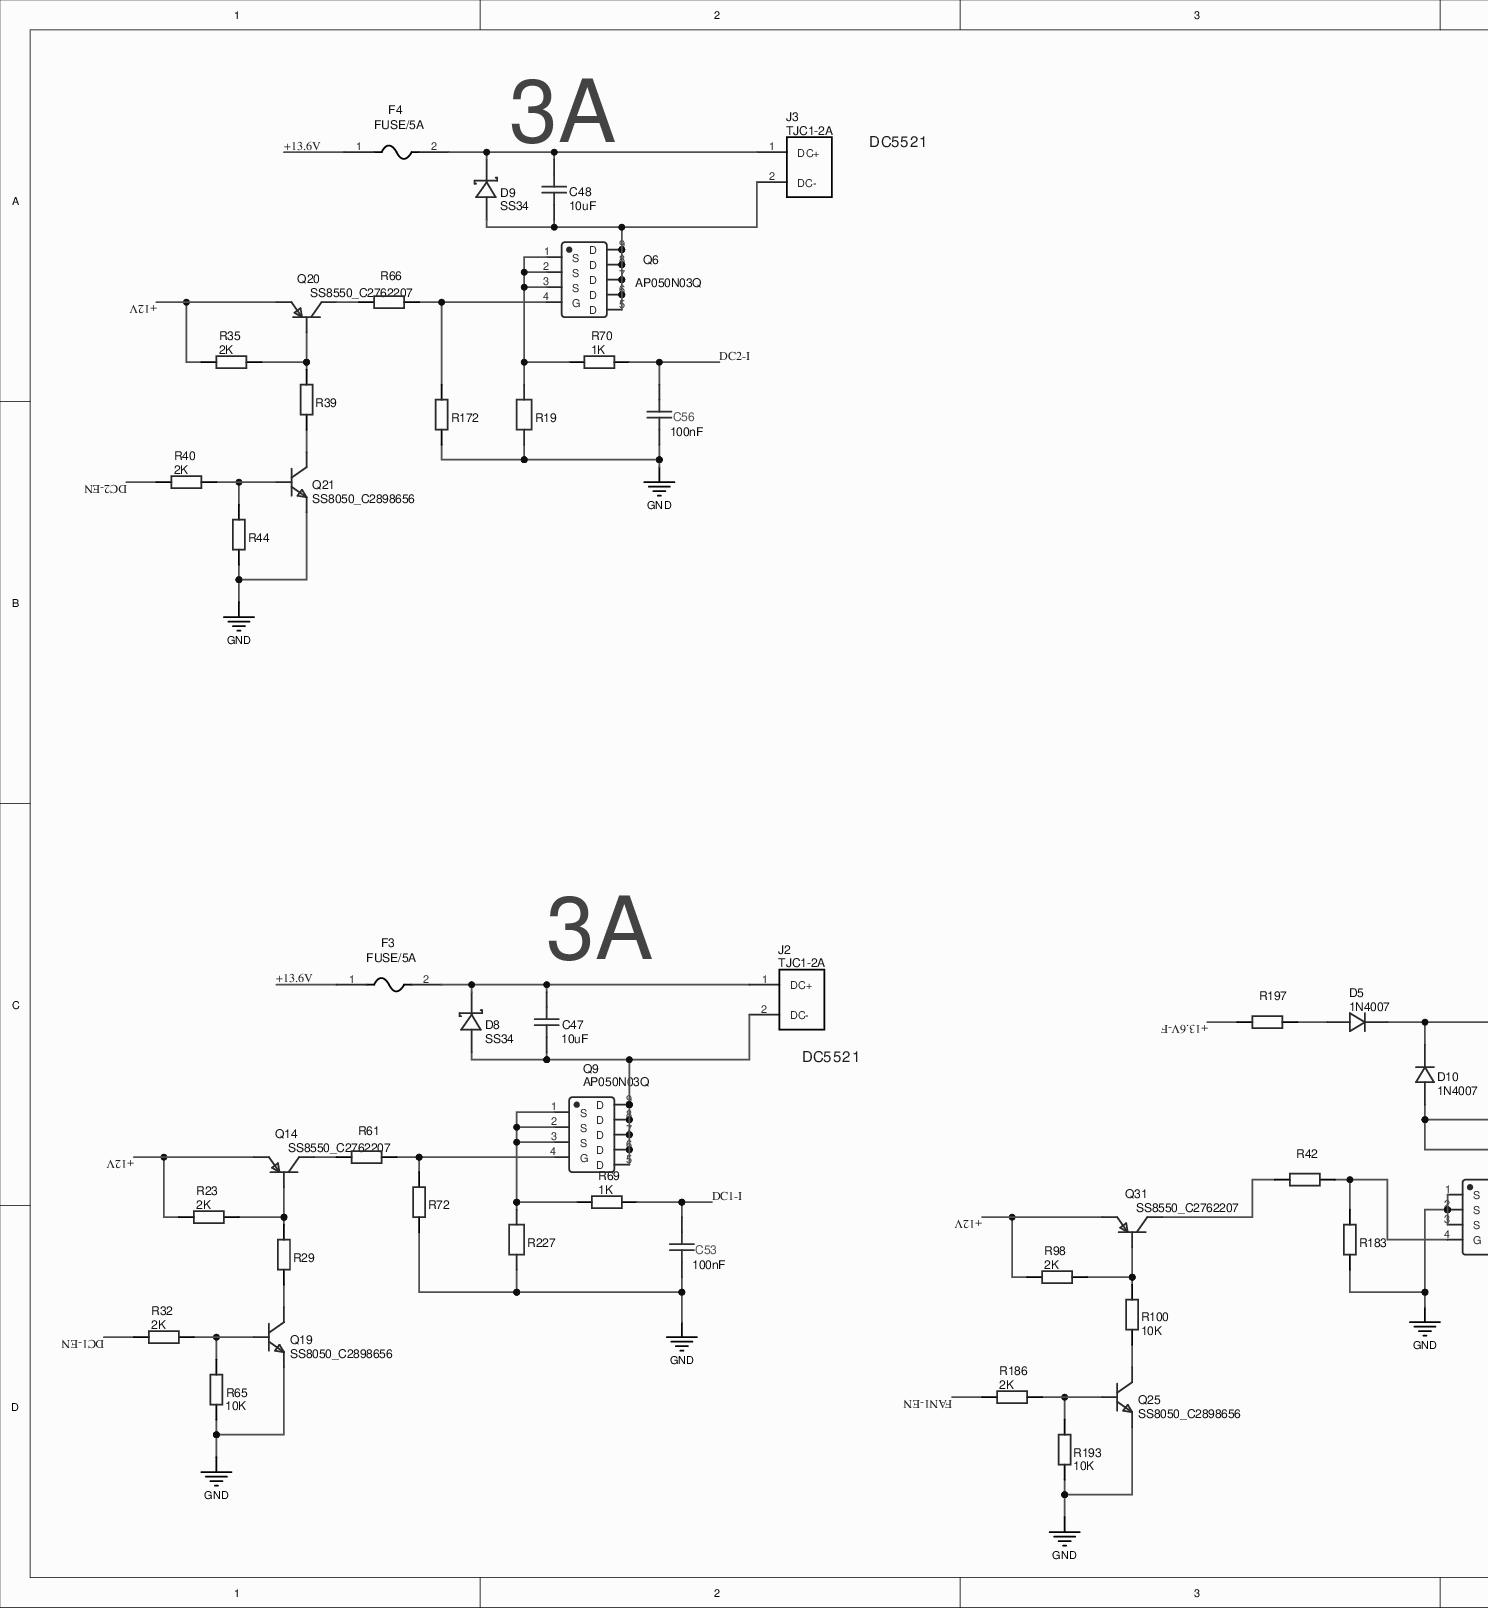
[diagram p0: MISC84402-8.SchDoc, left]
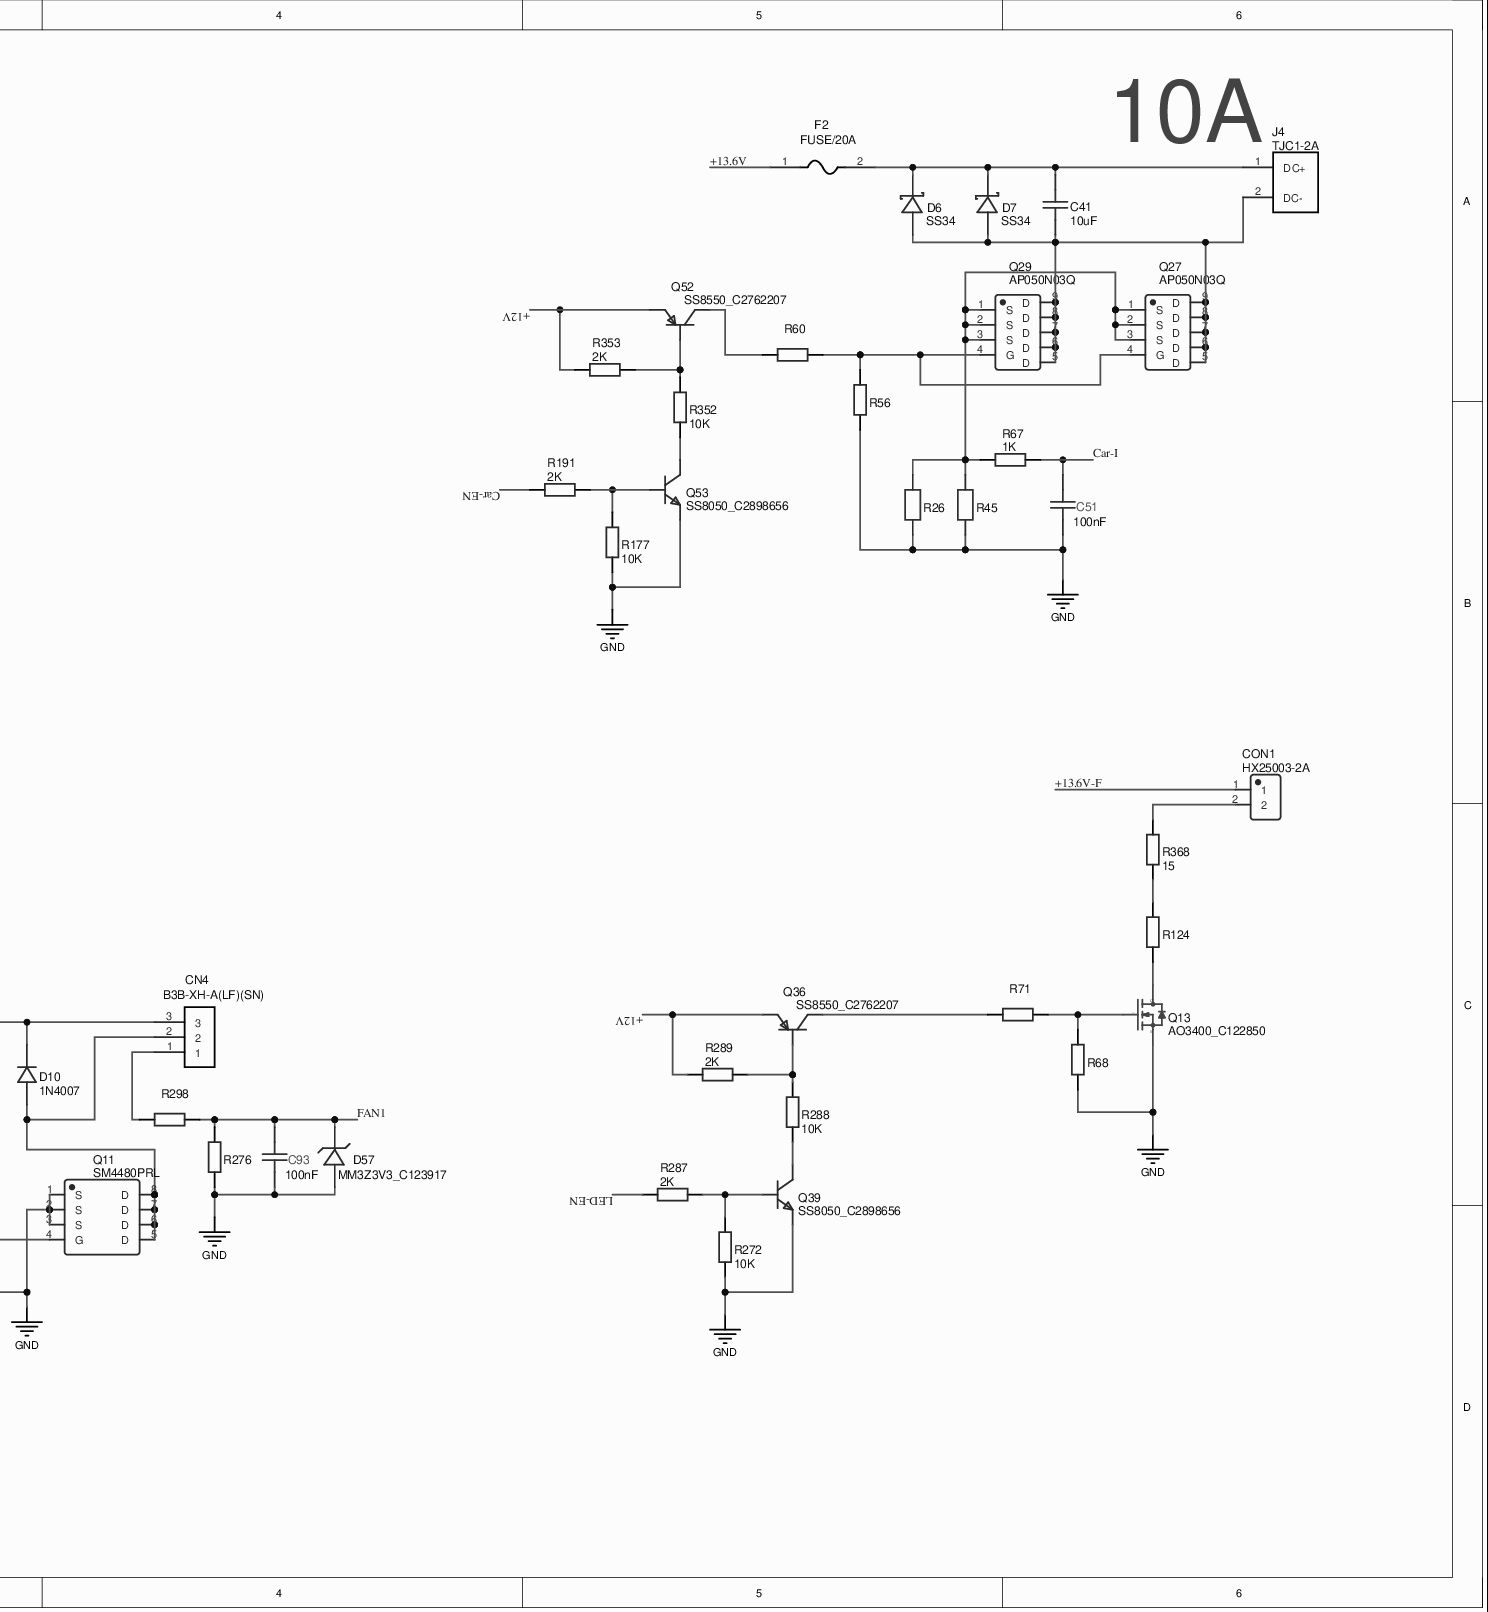
[diagram p1: MISC84402-8.SchDoc, right]
# Altium project MISC84402-4.PrjPcb (part 1 of 7)
8 sheets, 694 parts. Net scope: global (net labels, ports and power ports of the same name join across sheets).
Board file: MISC84402.PcbDoc
Sheets:
  MISC84402-8.SchDoc
  MISC84402-7.SchDoc
  MISC84402-10.SchDoc
  MISC84402-9.SchDoc
  MISC84402-11.SchDoc
  MISC84402-12.SchDoc
  MISC84402-5.SchDoc
  MISC84402-6.SchDoc

## Sheet MISC84402-8.SchDoc
size 487 x 272 mm

### Parts
C41  10uF  [C0603]
C47  10uF  [C0603]
C48  10uF  [C0603]
C51  100nF  [C0603]
C53  100nF  [C0603]
C56  100nF  [C0603]
C93  100nF  [C0603]
CN4  B3B-XH-A(LF)(SN)  [CONN-TH_3P-P2.50_B3B-XH-A-LF-SN]
CON1  HX25003-2A  [CONN-TH_2P-P2.50_HX25003-2A]
D5  1N4007  [DO-41_BD2.4-L4.7-P8.70-D0.9-RD]
D6  SS34  [SMC_L7.1-W6.2-LS8.1-R-RD]
D7  SS34  [SMC_L7.1-W6.2-LS8.1-R-RD]
D8  SS34  [SMC_L7.1-W6.2-LS8.1-R-RD]
D9  SS34  [SMC_L7.1-W6.2-LS8.1-R-RD]
D10  1N4007  [DO-41_BD2.4-L4.7-P8.70-D0.9-RD]
D57  MM3Z3V3_C123917  [SOD-323_L1.8-W1.3-LS2.5-RD]
F2  FUSE/20A  [FUSE-SMD_L6.1-W2.5]
F3  FUSE/5A  [FUSE-SMD_L6.1-W2.5]
F4  FUSE/5A  [FUSE-SMD_L6.1-W2.5]
J2  TJC1-2A  [DC5521]
J3  TJC1-2A  [DC5521]
J4  TJC1-2A  [CONN-TH_XT60UPB-F-W]
Q6  AP050N03Q  [PDFN-8_L3.1-W3.1-P0.65-LS3.4-BL]
Q9  AP050N03Q  [PDFN-8_L3.1-W3.1-P0.65-LS3.4-BL]
Q11  SM4480PRL  [SOP-8_L4.9-W3.9-P1.27-LS6.0-BL]
Q13  AO3400_C122850  [SC-59-3_L2.9-W1.5-P0.95-LS2.5-BR]
Q14  SS8550_C2762207  [SOT-23-3_L2.9-W1.3-P1.90-LS2.4-BR]
Q19  SS8050_C2898656  [SOT-23-3_L2.9-W1.3-P1.90-LS2.4-BR]
Q20  SS8550_C2762207  [SOT-23-3_L2.9-W1.3-P1.90-LS2.4-BR]
Q21  SS8050_C2898656  [SOT-23-3_L2.9-W1.3-P1.90-LS2.4-BR]
Q25  SS8050_C2898656  [SOT-23-3_L2.9-W1.3-P1.90-LS2.4-BR]
Q27  AP050N03Q  [PDFN-8_L3.1-W3.1-P0.65-LS3.4-BL]
Q29  AP050N03Q  [PDFN-8_L3.1-W3.1-P0.65-LS3.4-BL]
Q31  SS8550_C2762207  [SOT-23-3_L2.9-W1.3-P1.90-LS2.4-BR]
Q36  SS8550_C2762207  [SOT-23-3_L2.9-W1.3-P1.90-LS2.4-BR]
Q39  SS8050_C2898656  [SOT-23-3_L2.9-W1.3-P1.90-LS2.4-BR]
Q52  SS8550_C2762207  [SOT-23-3_L2.9-W1.3-P1.90-LS2.4-BR]
Q53  SS8050_C2898656  [SOT-23-3_L2.9-W1.3-P1.90-LS2.4-BR]
R19  (no value)  [RES-SMD_L6.4-W3.2-R2512]
R23  2K  [R0603]
R26  (no value)  [R2512]
R29  (no value)  [R0603]
R32  2K  [R0603]
R35  2K  [R0603]
R39  (no value)  [R0603]
R40  2K  [R0603]
R42  (no value)  [R0603]
R44  (no value)  [R0603]
R45  (no value)  [R2512]
R56  (no value)  [R0603]
R60  (no value)  [R0603]
R61  (no value)  [R0603]
R65  10K  [R0603]
R66  (no value)  [R0603]
R67  1K  [R0603]
R68  (no value)  [R0603]
R69  1K  [R0603]
R70  1K  [R0603]
R71  (no value)  [R0603]
R72  (no value)  [R0603]
R98  2K  [R0603]
R100  10K  [R0603]
R124  (no value)  [R0603]
R172  (no value)  [R0603]
R177  10K  [R0603]
R183  (no value)  [R0603]
R186  2K  [R0603]
R191  2K  [R0603]
R193  10K  [R0603]
R197  (no value)  [R0603]
R227  (no value)  [RES-SMD_L6.4-W3.2-R2512]
R272  10K  [R0603]
R276  (no value)  [R0603]
R287  2K  [R0603]
R288  10K  [R0603]
R289  2K  [R0603]
R298  (no value)  [R0603]
R352  10K  [R0603]
R353  2K  [R0603]
R368  15  [r2512]

### Nets
GND: C51.1 C53.1 C56.1 C93.1 D57.2(A) Q11.1(S) Q11.2(S) Q11.3(S) Q13.2(S) Q19.2(E) Q21.2(E) Q25.2(E) Q39.2(E) Q53.2(E) R19.1 R26.1 R44.2 R45.1 R56.1 R65.2 R68.1 R72.2 R172.1 R177.2 R183.1 R193.2 R227.1 R272.2 R276.1
+12V: Q14.2(E) Q20.2(E) Q31.2(E) Q36.2(E) Q52.2(E) R23.1 R35.1 R98.1 R289.1 R353.1
+13.6V: F2.1 F3.1 F4.1
+13.6V-F: CON1.1 R197.1
Car-EN: R191.1
Car-I: C51.2 R67.2
DC1-EN: R32.1
DC1-I: C53.2 R69.2
DC2-EN: R40.1
DC2-I: C56.2 R70.2
FAN1: C93.2 D57.1(K) R276.2 R298.2
FAN1-EN: R186.1
LED-EN: R287.1
NetC41_1: C41.1 D6.1(A) D7.1(A) J4.2(DC-) Q27.5(D) Q27.6(D) Q27.7(D) Q27.8(D) Q27.9(D) Q29.5(D) Q29.6(D) Q29.7(D) Q29.8(D) Q29.9(D)
NetC41_2: C41.2 D6.2(K) D7.2(K) F2.2 J4.1(DC+)
NetC47_1: C47.1 D8.1(A) J2.2(DC-) Q9.5(D) Q9.6(D) Q9.7(D) Q9.8(D) Q9.9(D)
NetC47_2: C47.2 D8.2(K) F3.2 J2.1(DC+)
NetC48_1: C48.1 D9.1(A) J3.2(DC-) Q6.5(D) Q6.6(D) Q6.7(D) Q6.8(D) Q6.9(D)
NetC48_2: C48.2 D9.2(K) F4.2 J3.1(DC+)
NetCN4_1: CN4.1 R298.1
NetCN4_2: CN4.2 D10.2 Q11.5(D) Q11.6(D) Q11.7(D) Q11.8(D)
NetCN4_3: CN4.3 D5.1 D10.1
NetCON1_2: CON1.2 R368.2
NetD5_2: D5.2 R197.2
NetQ6_1: Q6.1(S) Q6.2(S) Q6.3(S) R19.2 R70.1
NetQ6_4: Q6.4(G) R66.2 R172.2
NetQ9_1: Q9.1(S) Q9.2(S) Q9.3(S) R69.1 R227.2
NetQ9_4: Q9.4(G) R61.2 R72.1
NetQ11_4: Q11.4(G) R42.2 R183.2
NetQ13_1: Q13.1(G) R68.2 R71.2
NetQ13_3: Q13.3(D) R124.1
NetQ14_1: Q14.1(B) R23.2 R29.1
NetQ14_3: Q14.3(C) R61.1
NetQ19_1: Q19.1(B) R32.2 R65.1
NetQ19_3: Q19.3(C) R29.2
NetQ20_1: Q20.1(B) R35.2 R39.1
NetQ20_3: Q20.3(C) R66.1
NetQ21_1: Q21.1(B) R40.2 R44.1
NetQ21_3: Q21.3(C) R39.2
NetQ25_1: Q25.1(B) R186.2 R193.1
NetQ25_3: Q25.3(C) R100.1
NetQ27_1: Q27.1(S) Q27.2(S) Q27.3(S) Q29.1(S) Q29.2(S) Q29.3(S) R26.2 R45.2 R67.1
NetQ27_4: Q27.4(G) Q29.4(G) R56.2 R60.2
NetQ31_1: Q31.1(B) R98.2 R100.2
NetQ31_3: Q31.3(C) R42.1
NetQ36_1: Q36.1(B) R288.2 R289.2
NetQ36_3: Q36.3(C) R71.1
NetQ39_1: Q39.1(B) R272.1 R287.2
NetQ39_3: Q39.3(C) R288.1
NetQ52_1: Q52.1(B) R352.2 R353.2
NetQ52_3: Q52.3(C) R60.1
NetQ53_1: Q53.1(B) R177.1 R191.2
NetQ53_3: Q53.3(C) R352.1
NetR124_2: R124.2 R368.1

### Notes on the sheet
- (near C48) 3A
- DC5521
- (near J4) 10A
- (near C47) 3A
- (near J2) DC5521

### Library data of the parts
C41 C47 C48 = 10uF: BOM_Manufacturer: FH(Guangdong Fenghua Advanced Tech); BOM_Manufacturer Part: 0603X106M250NT; nameAlias: Capacitance; Contributor: LCSC; BOM_Supplier: LCSC; BOM_Supplier Part: C479655; BOM_JLCPCB Part Class: Extended Part; spicePre: C; spiceSymbolName: 0603X106M250NT
C51 C53 C56 C93 = 100nF: BOM_Manufacturer: SAMSUNG; BOM_Manufacturer Part: CL10B104KC8NNNC; nameAlias: Capacitance; BOM_Supplier: LCSC; BOM_Supplier Part: C15725; BOM_JLCPCB Part Class: Extended Part; spicePre: C; spiceSymbolName: CL10B104KC8NNNC
CN4 = B3B-XH-A(LF)(SN): BOM_Manufacturer: JST Sales America; Contributor: LCSC; BOM_Supplier: LCSC; BOM_Supplier Part: C144394; BOM_Manufacturer Part: B3B-XH-A(LF)(SN); BOM_JLCPCB Part Class: Extended Part; spicePre: U; spiceSymbolName: B3B-XH-A(LF)(SN)
CON1 = HX25003-2A: BOM_Manufacturer: HX(Zhejiang Yueqing Hongxing Elec); Contributor: LCSC; BOM_Supplier: LCSC; BOM_Supplier Part: C442299; BOM_Manufacturer Part: HX25003-2A; BOM_JLCPCB Part Class: Extended Part; spicePre: C; spiceSymbolName: HX25003-2A
D5 D10 = 1N4007: BOM_Manufacturer: SEMTECH; Contributor: LCEDA_Lib; BOM_Supplier: LCSC; BOM_Manufacturer Part: 1N4007; BOM_Supplier Part: C106903; spicePre: D; spiceSymbolName: 1N4007
D6-D9 = SS34: BOM_Manufacturer: MDD; BOM_Supplier: LCSC; BOM_Manufacturer Part: SS34; BOM_Supplier Part: C13763; BOM_JLCPCB Part Class: Extended Part; spicePre: D; spiceSymbolName: SS34
D57 = MM3Z3V3_C123917: BOM_Manufacturer: Shandong Jingdao Microelectronics; Contributor: LCSC; BOM_Supplier: LCSC; BOM_Supplier Part: C123917; BOM_Manufacturer Part: MM3Z3V3; BOM_JLCPCB Part Class: Extended Part; spicePre: D; spiceSymbolName: MM3Z3V3_C123917
F2 = FUSE/20A: BOM_Manufacturer: RUILON; BOM_Supplier: LCSC; BOM_Supplier Part: C30198; BOM_JLCPCB Part Class: Extended Part; spicePre: F
F3 F4 = FUSE/5A: BOM_Manufacturer: RUILON; BOM_Supplier: LCSC; BOM_Supplier Part: C30198; BOM_JLCPCB Part Class: Extended Part; spicePre: F
J2-J4 = TJC1-2A: BOM_Manufacturer: ReliaPro; BOM_Supplier: LCSC; BOM_Manufacturer Part: TJC1-2A; BOM_Supplier Part: C29632; spicePre: J; spiceSymbolName: TJC1-2A
Q6 Q9 Q27 Q29 = AP050N03Q: Contributor: LCSC; BOM_Supplier: LCSC; BOM_Supplier Part: C471915; BOM_Manufacturer Part: AP050N03Q; BOM_JLCPCB Part Class: Extended Part; spicePre: Q; spiceSymbolName: AP050N03Q
Q11 = SM4480PRL: BOM_Manufacturer: SPS; Contributor: LCSC; BOM_Supplier: LCSC; BOM_Supplier Part: C350659; BOM_Manufacturer Part: SM4480PRL; BOM_JLCPCB Part Class: Extended Part; spicePre: Q; spiceSymbolName: SM4480PRL
Q13 = AO3400_C122850: BOM_Manufacturer: SK; BOM_Manufacturer Part: AO3400; BOM_Supplier: LCSC; BOM_Supplier Part: C122850; BOM_JLCPCB Part Class: Extended Part; spicePre: Q; spiceSymbolName: AO3400_C122850
Q14 Q20 Q31 Q36 Q52 = SS8550_C2762207: BOM_Manufacturer Part: SS8550; Contributor: LCSC; BOM_Supplier: LCSC; BOM_Supplier Part: C2762207; BOM_JLCPCB Part Class: Extended Part; spicePre: Q; spiceSymbolName: SS8550_C2762207
Q19 Q21 Q25 Q39 Q53 = SS8050_C2898656: BOM_Manufacturer Part: SS8050; Contributor: LCSC; BOM_Supplier: LCSC; BOM_Supplier Part: C2898656; spicePre: Q; spiceSymbolName: SS8050_C2898656
R19 R227 = (no symbol name): BOM_Manufacturer Part: HoJLR2512-3W-50mR-1%; nameAlias: Resistance; Contributor: lcsc; BOM_Supplier: LCSC; BOM_Supplier Part: C2903475; BOM_JLCPCB Part Class: Extended Part; spicePre: R; spiceSymbolName: HOJLR2512-3W-50MR-1%
R23 R32 R35 R40 R98 R186 R191 R287 R289 R353 = 2K: BOM_Manufacturer: UniOhm; BOM_Manufacturer Part: 0603WAF2001T5E; nameAlias: Resistance (Ohms); BOM_Supplier: LCSC; BOM_Supplier Part: C22975; BOM_JLCPCB Part Class: Basic Part; spicePre: R; spiceSymbolName: 0603WAF2001T5E
R26 R45 = (no symbol name): BOM_Manufacturer: Milliohm; BOM_Manufacturer Part: GX2512-2W-20mR-1%; Resistance (Ohms): 0.02; nameAlias: Resistance; Contributor: LCSC; BOM_Supplier: LCSC; BOM_Supplier Part: C500720; BOM_JLCPCB Part Class: Extended Part; spicePre: R; spiceSymbolName: GX2512-2W-20MR-1%
R29 R39 R44 = (no symbol name): BOM_Manufacturer: UniOhm; BOM_Manufacturer Part: 0603WAF1002T5E; nameAlias: Resistance; Resistance (Ohms): 10K; BOM_Supplier: LCSC; BOM_Supplier Part: C25804; BOM_JLCPCB Part Class: Basic Part; spicePre: R; spiceSymbolName: 0603WAF1002T5E
R42 R60 R61 R66 R71 = (no symbol name): BOM_Manufacturer: UniOhm; BOM_Manufacturer Part: 0603WAF100JT5E; nameAlias: Resistance; BOM_Supplier: LCSC; BOM_Supplier Part: C22859; BOM_JLCPCB Part Class: Basic Part; spicePre: R; spiceSymbolName: 0603WAF100JT5E
R56 R68 R72 R172 R183 = (no symbol name): BOM_Manufacturer: UniOhm; BOM_Manufacturer Part: 0603WAF3002T5E; nameAlias: Resistance; Resistance (Ohms): 30K; BOM_Supplier: LCSC; BOM_Supplier Part: C22984; BOM_JLCPCB Part Class: Basic Part; spicePre: R; spiceSymbolName: 0603WAF3002T5E
R65 R100 R177 R193 R272 R288 R352 = 10K: BOM_Manufacturer: FH; BOM_Manufacturer Part: RS-03K102JT; nameAlias: Resistance (Ohms); BOM_Supplier: LCSC; BOM_Supplier Part: C73797; spicePre: R; spiceSymbolName: RS-03K102JT
R67 R69 R70 = 1K: BOM_Manufacturer: FH; BOM_Manufacturer Part: RS-03K102JT; nameAlias: Resistance (Ohms); BOM_Supplier: LCSC; BOM_Supplier Part: C73797; spicePre: R; spiceSymbolName: RS-03K102JT
R124 R197 = (no symbol name): BOM_Manufacturer: UniOhm; BOM_Manufacturer Part: 0603WAF0000T5E; nameAlias: Resistance; Resistance (Ohms): 0; BOM_Supplier: LCSC; BOM_Supplier Part: C21189; BOM_JLCPCB Part Class: Basic Part; spicePre: R; spiceSymbolName: 0603WAF0000T5E
R276 = (no symbol name): BOM_Manufacturer: UniOhm; BOM_Manufacturer Part: 0603WAF2001T5E; nameAlias: Resistance; Resistance (Ohms): 2K; BOM_Supplier: LCSC; BOM_Supplier Part: C22975; BOM_JLCPCB Part Class: Basic Part; spicePre: R; spiceSymbolName: 0603WAF2001T5E
R298 = (no symbol name): BOM_Manufacturer: UniOhm; BOM_Manufacturer Part: 0603WAF5601T5E; nameAlias: Resistance; Resistance (Ohms): 5.6K; BOM_Supplier: LCSC; BOM_Supplier Part: C23189; BOM_JLCPCB Part Class: Basic Part; spicePre: R; spiceSymbolName: 0603WAF5601T5E
R368 = 15: BOM_Manufacturer: UniOhm; BOM_Manufacturer Part: MFR02SF150JA10; nameAlias: Resistance (Ohms); BOM_Supplier: LCSC; BOM_Supplier Part: C63443; BOM_JLCPCB Part Class: Extended Part; spicePre: R; spiceSymbolName: MFR02SF150JA10

## Sheet MISC84402-7.SchDoc
size 534 x 349 mm
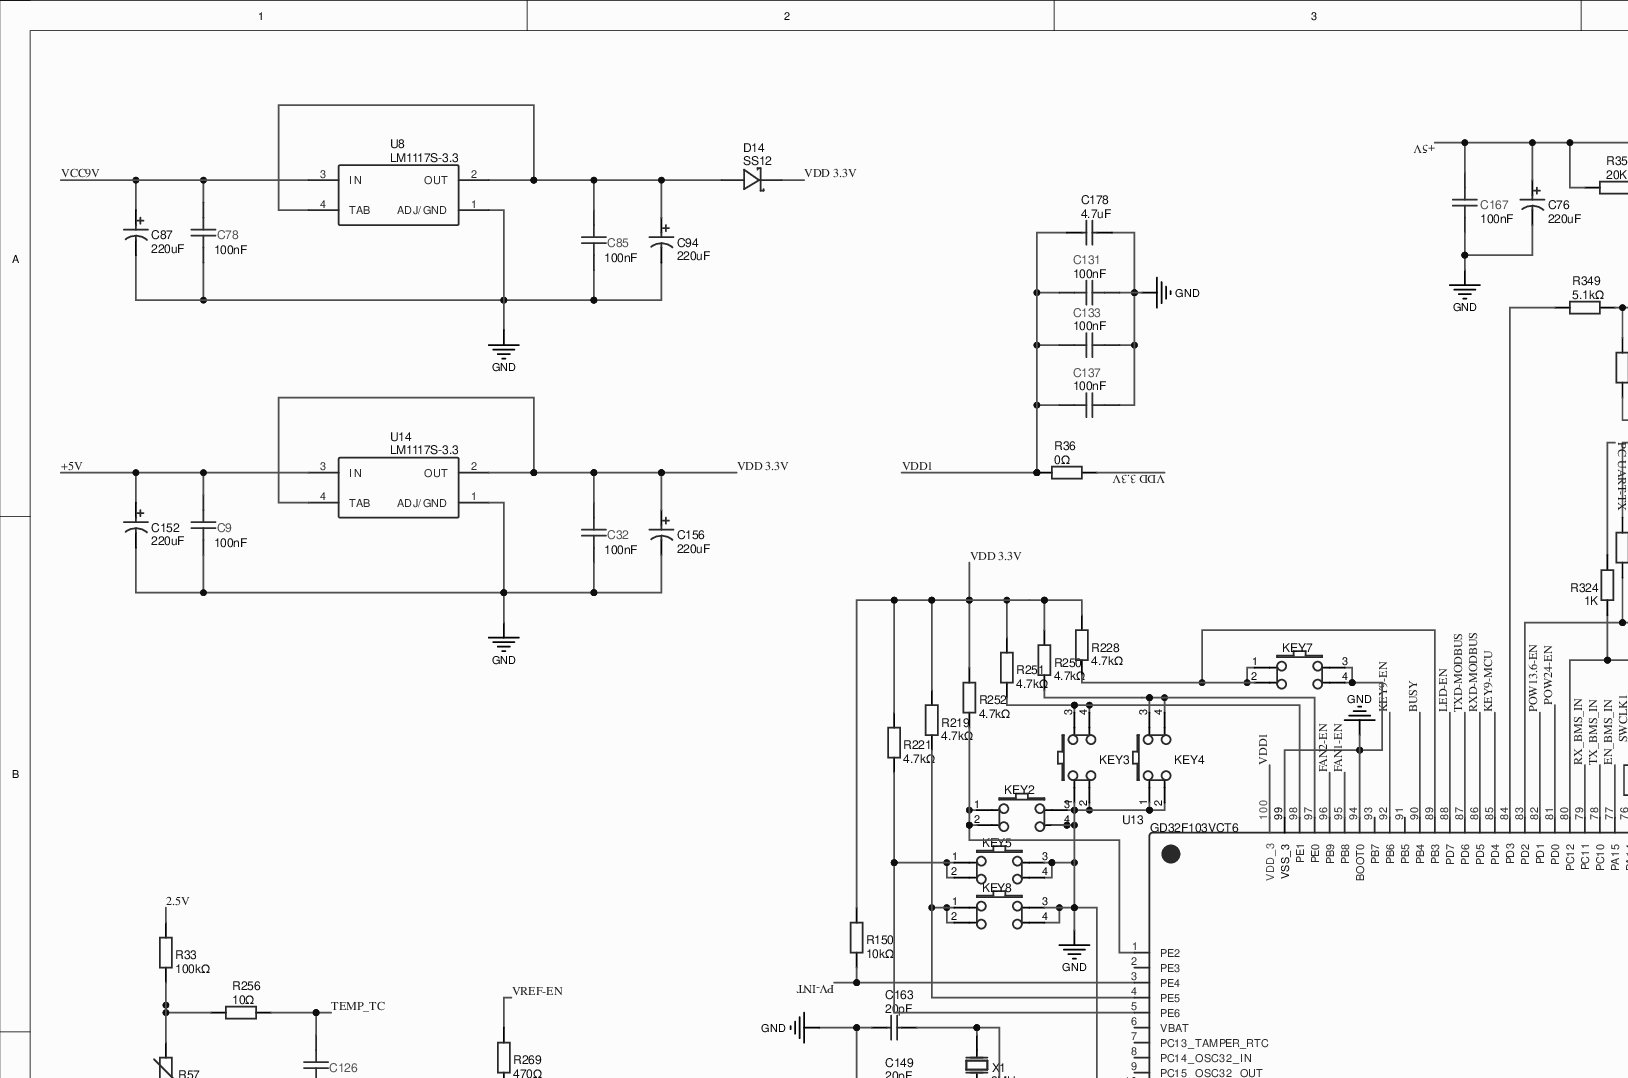
[diagram p2: MISC84402-7.SchDoc, top left]
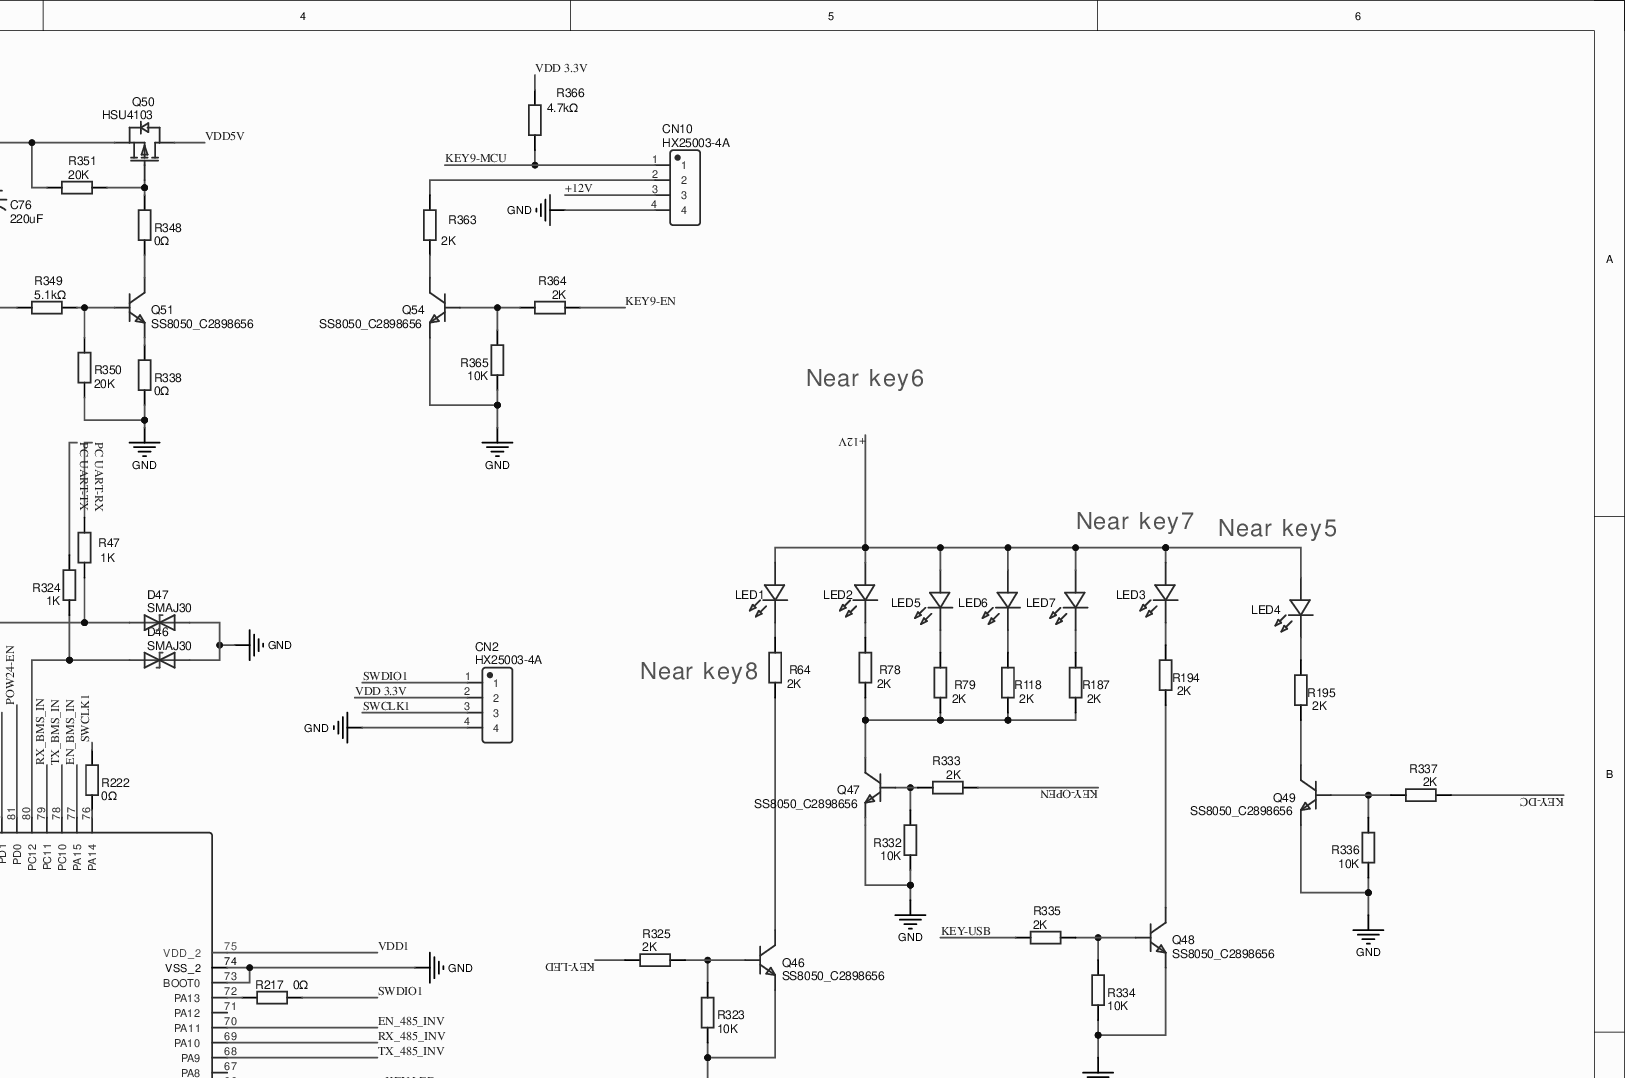
[diagram p3: MISC84402-7.SchDoc, top right]
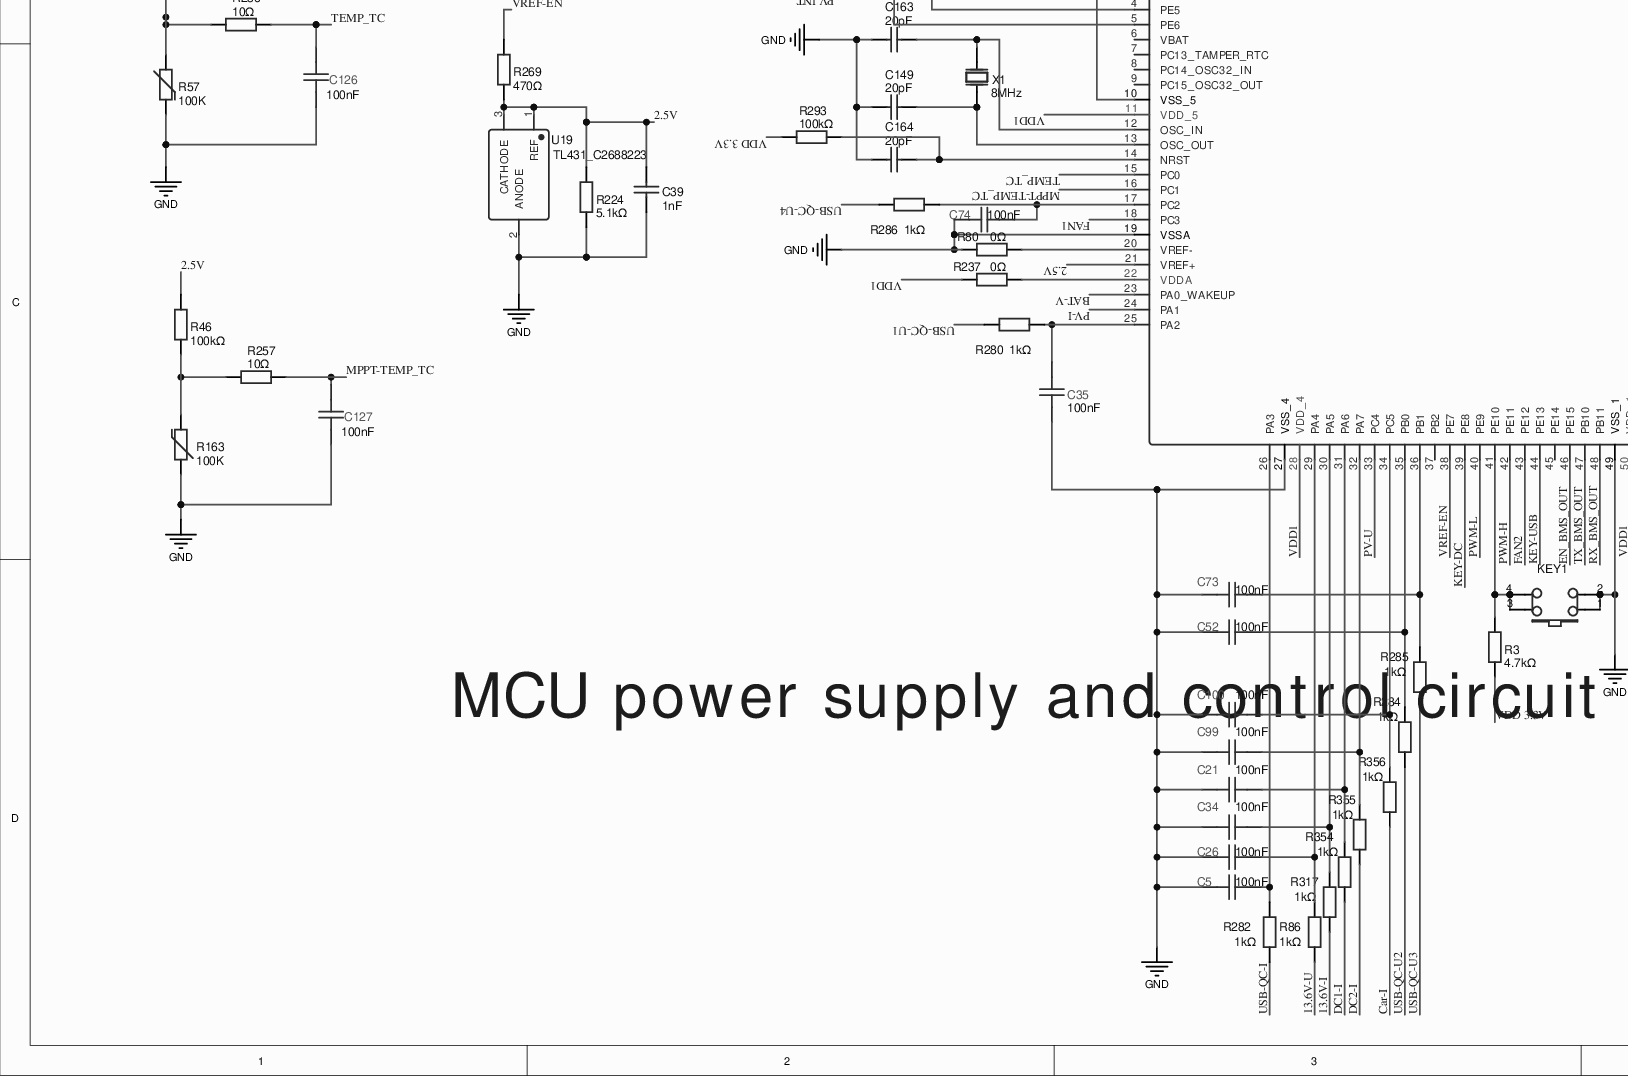
[diagram p4: MISC84402-7.SchDoc, bottom left]
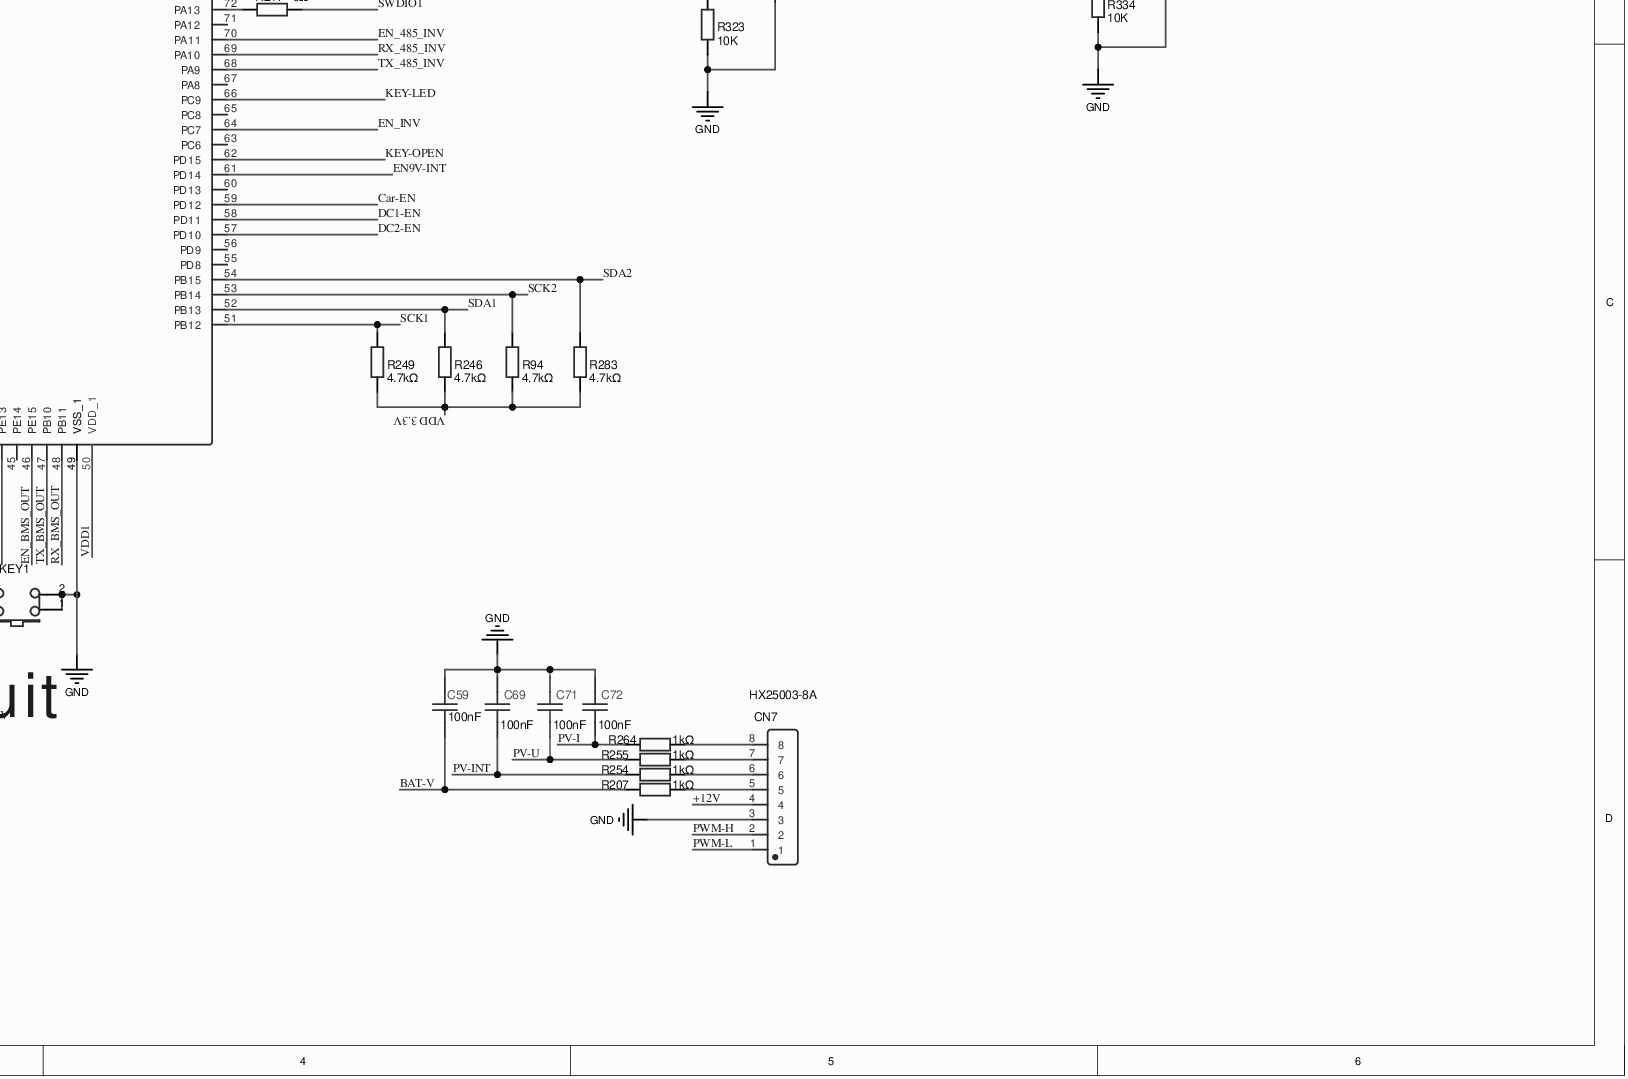
[diagram p5: MISC84402-7.SchDoc, bottom right]

### Parts
C5  100nF  [C0603]